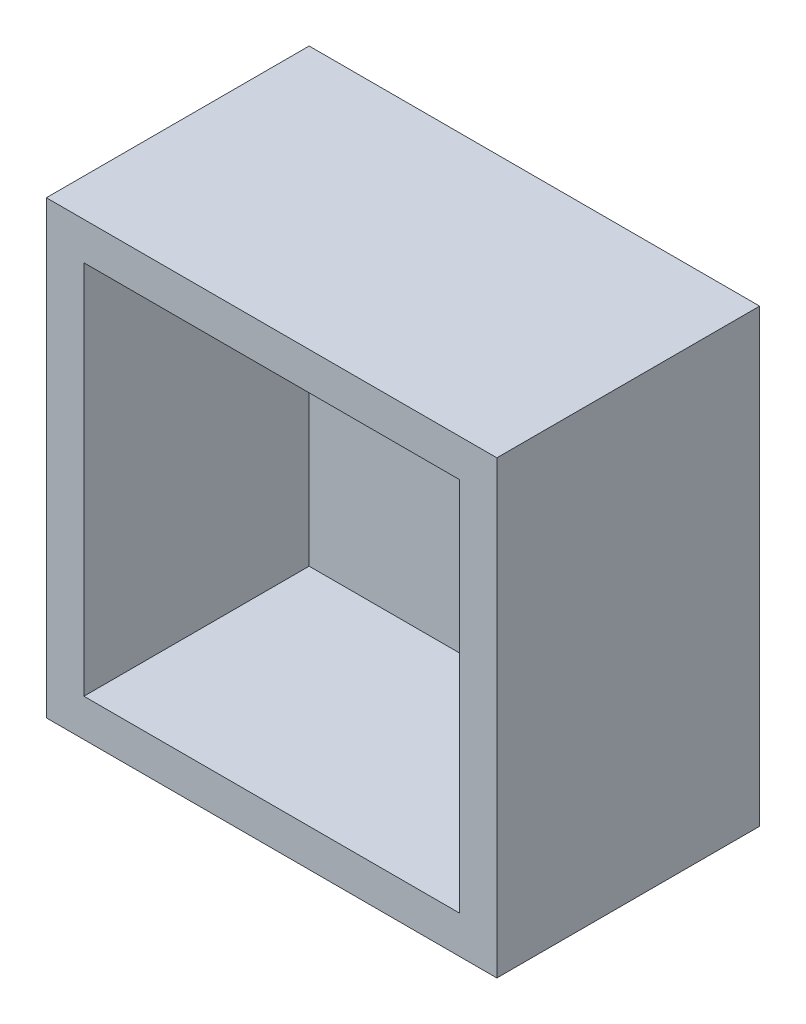
SolidWorks part; units mm, degrees
ref_plane "Front Plane" through (0, 0, 0) normal (0, 0, 1) x (1, 0, 0)
ref_plane "Top Plane" through (0, 0, 0) normal (0, 1, 0) x (1, 0, 0)
ref_plane "Right Plane" through (0, 0, 0) normal (1, 0, 0) x (0, 0, -1)
sketch "Sketch1" plane through (0, 0, 0) normal (0, 0, 1) x (1, 0, 0)
  line L0 (0, 0) -> (-88, 0) construction
  line L1 (-130, -85) -> (-130, 85) construction
  line L2 (-118, 30) -> (-58, 30)
  line L3 (-118, 30) -> (-118, -30)
  line L4 (-118, -30) -> (-58, -30)
  line L5 (-58, 30) -> (-58, -30)
  line L6 (-118, 30) -> (-58, -30) construction
  line L7 (-118, -30) -> (-58, 30) construction
  dimension "D1" = 60
  dimension "D2" = 60
  dimension "D3" = 12
extrude "Boss-Extrude1" add sketch "Sketch1" along normal blind 35
shell "Shell1" thickness 5
